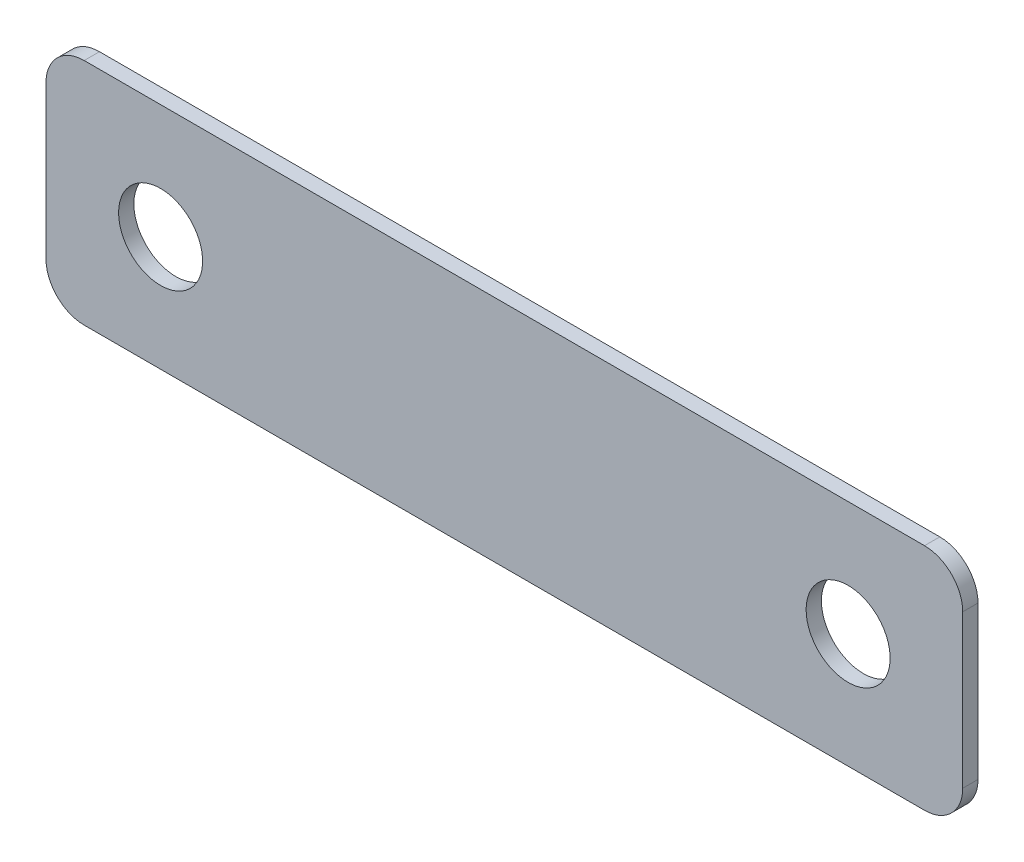
SolidWorks part; units mm, degrees
ref_plane "前视基准面" through (0, 0, 0) normal (0, 0, 1) x (1, 0, 0)
ref_plane "上视基准面" through (0, 0, 0) normal (0, 1, 0) x (1, 0, 0)
ref_plane "右视基准面" through (0, 0, 0) normal (1, 0, 0) x (0, 0, -1)
sketch "草图1" plane through (0, 0, 0) normal (0, 0, 1) x (1, 0, 0)
  line L1 (-60, -15) -> (60, -15)
  line L2 (-60, -15) -> (-60, 15)
  line L3 (-60, 15) -> (60, 15)
  line L4 (60, -15) -> (60, 15)
  line L5 (-60, -15) -> (60, 15) construction
  line L6 (-60, 15) -> (60, -15) construction
  point P0 (0, 0)
  dimension "D1" = 30
  dimension "D2" = 120
extrude "凸台-拉伸1" add sketch "草图1" along normal blind 2
sketch "草图2" plane through (0, 0, 0) normal (0, 0, -1) x (-1, 0, 0)
  line L0 (0, 0) -> (53.1143, 0) construction
  line L1 (53.1143, 0) -> (-53.8661, 0) construction
  line L3 (0, 0) -> (0, -22.8345) construction
  circle A0 centre (45, 0) radius 5.5
  circle A1 centre (-45, 0) radius 5.5
  dimension "D1" = 11
  dimension "D2" = 90
extrude "切除-拉伸1" cut sketch "草图2" against normal blind 10
fillet "圆角1" radius 5 4 edges at (-60, -15, 1) (-60, 15, 1) (60, -15, 1) (60, 15, 1)
